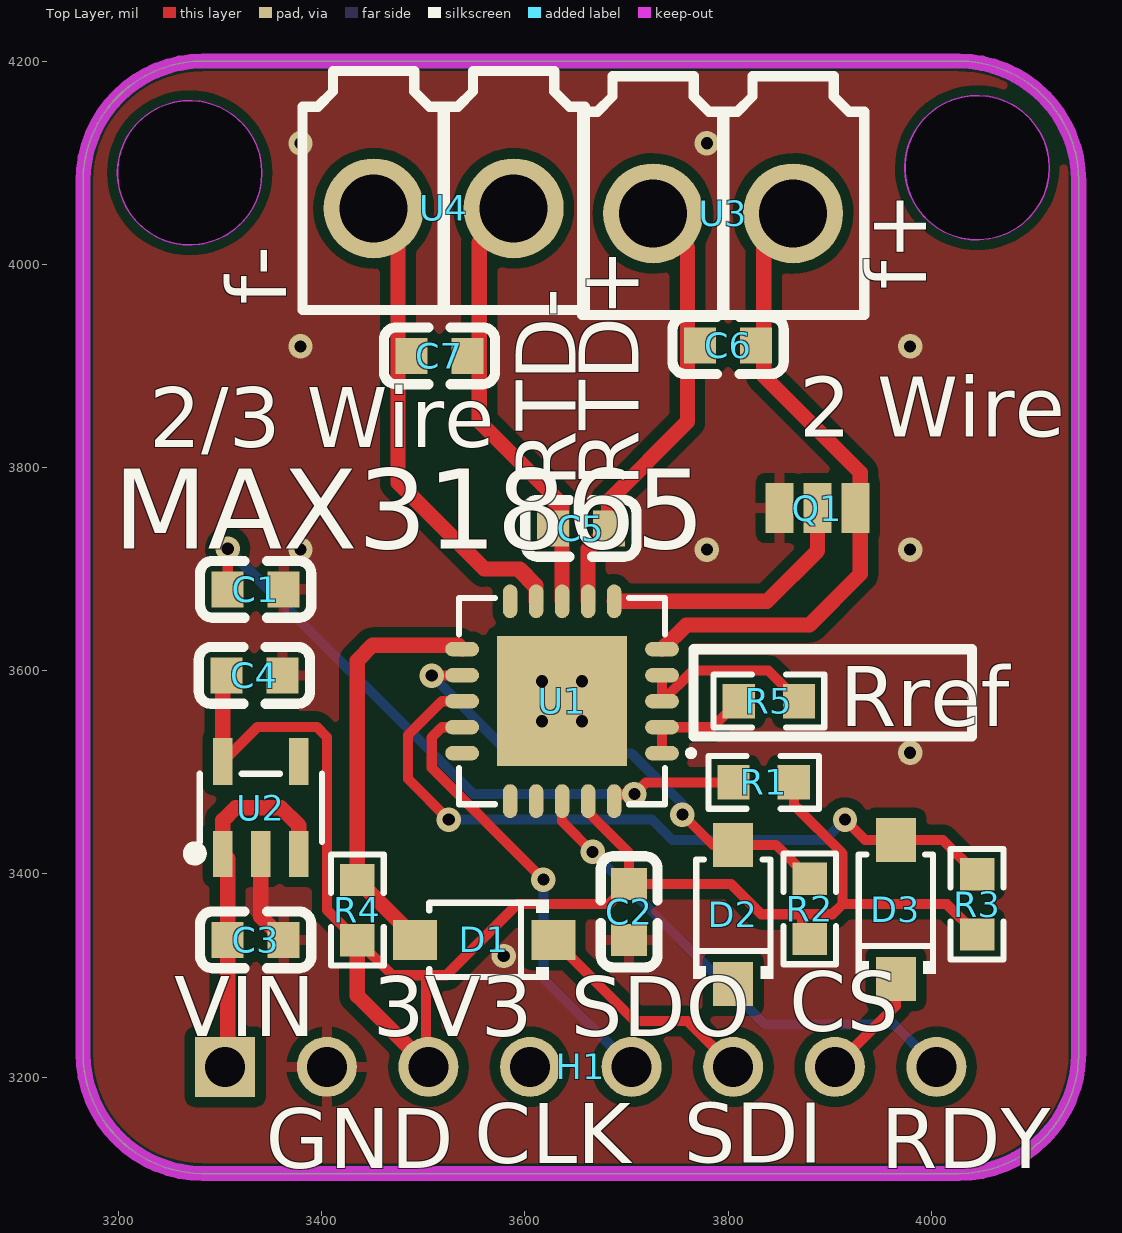
[diagram p0: Top Layer view]
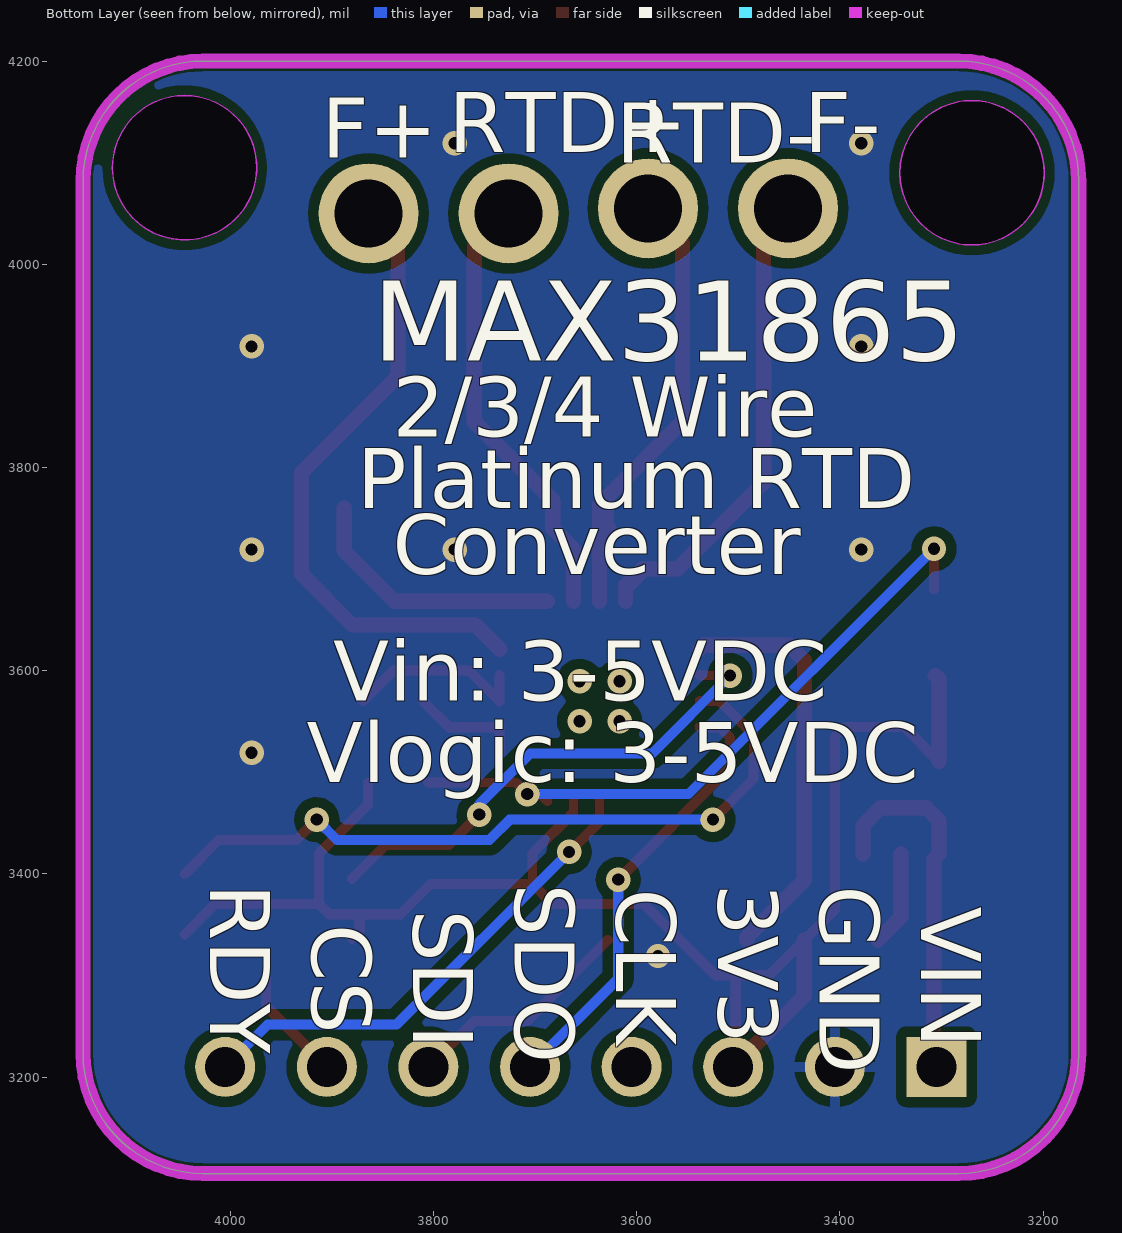
[diagram p1: Bottom Layer view, seen from below]
# Altium PCB MISC82906.pcbdoc
Units mil, origin at the board's own origin, x right, y up, seen from the top; angles counter-clockwise.
Board outline 980 x 1095 mil, 2 copper layers (Top Layer, Bottom Layer), stack 62.206 mil thick; 21 components, 20 nets, 71 pads, 21 vias.

## Layer stack, top to bottom
Top Solder Mask Layer: solder mask 0.394, Dk 3.3
Top Layer: signal copper 1.379
Dielectric1: surface 59.449, FR4, Dk 4.5
Bottom Layer: signal copper 1.378
Bottom Solder Mask Layer: solder mask 0.394, Dk 3.3

## Board outline
3283.11,4200 ccw(c3283.11,4081.89) 3165,4081.89 3165,3223.11 ccw(c3283.11,3223.11) 3283.11,3105 4026.89,3105 ccw(c4026.89,3223.11) 4145,3223.11 4145,4081.89 ccw(c4026.89,4081.89) 4026.89,4200
cut-out: 3341.06,4090 cw(c3270,4090) 3198.94,4090 cw(c3270,4090)
cut-out: 4116.06,4095 cw(c4045,4095) 3973.94,4095 cw(c4045,4095)

## Design rules (kind name [scope] priority, off if disabled: settings)
BoardOutlineClearance copperThickness2oz_1 [All] p2 off: genericclearance=7.99 ignorepadtopadclearanceinfootprint=FALSE except(0: Arc-SplitContinuation Track-SplitContinuation SMDPad-SplitContinuation THPad-SplitContinuation Via-SplitContinuation Fill-SplitContinuation Region-SplitContinuation Poly-SplitContinuation Text-SplitContinuation Hole-SplitContinuation; 5.98: Arc-CutoutEdge Track-CutoutEdge SMDPad-CutoutEdge THPad-CutoutEdge Via-CutoutEdge Text-CutoutEdge; 6.9: Hole-OutlineEdge Hole-CutoutEdge; 10: Poly-OutlineEdge Poly-CutoutEdge; 11.81: Arc-OutlineEdge Track-OutlineEdge SMDPad-OutlineEdge THPad-OutlineEdge Via-OutlineEdge Fill-OutlineEdge Region-OutlineEdge Text-OutlineEdge Fill-CutoutEdge Region-CutoutEdge)
BoardOutlineClearance Plane_innerPlane_1 [All] p4 off: genericclearance=4.02 ignorepadtopadclearanceinfootprint=FALSE except(0: Arc-SplitContinuation Track-SplitContinuation SMDPad-SplitContinuation THPad-SplitContinuation Via-SplitContinuation Fill-SplitContinuation Region-SplitContinuation Poly-SplitContinuation Text-SplitContinuation Hole-SplitContinuation; 5.98: Arc-CutoutEdge Track-CutoutEdge SMDPad-CutoutEdge THPad-CutoutEdge Via-CutoutEdge Text-CutoutEdge; 6.9: Hole-OutlineEdge Hole-CutoutEdge; 10: Poly-OutlineEdge Poly-CutoutEdge; 11.81: Arc-OutlineEdge Track-OutlineEdge SMDPad-OutlineEdge THPad-OutlineEdge Via-OutlineEdge Fill-OutlineEdge Region-OutlineEdge Text-OutlineEdge Fill-CutoutEdge Region-CutoutEdge)
BoardOutlineClearance Copper_copperRegion_1 [All] p6 off: genericclearance=4.02 ignorepadtopadclearanceinfootprint=FALSE except(0: Arc-SplitContinuation Track-SplitContinuation SMDPad-SplitContinuation THPad-SplitContinuation Via-SplitContinuation Fill-SplitContinuation Region-SplitContinuation Poly-SplitContinuation Text-SplitContinuation Hole-SplitContinuation; 5.98: Arc-CutoutEdge Track-CutoutEdge SMDPad-CutoutEdge THPad-CutoutEdge Via-CutoutEdge Text-CutoutEdge; 6.9: Hole-OutlineEdge Hole-CutoutEdge; 10: Poly-OutlineEdge Poly-CutoutEdge; 11.81: Arc-OutlineEdge Track-OutlineEdge SMDPad-OutlineEdge THPad-OutlineEdge Via-OutlineEdge Fill-OutlineEdge Region-OutlineEdge Text-OutlineEdge Fill-CutoutEdge Region-CutoutEdge)
BoardOutlineClearance copperThickness1oz_1 [All] p8: genericclearance=4.02 ignorepadtopadclearanceinfootprint=FALSE except(0: Arc-SplitContinuation Track-SplitContinuation SMDPad-SplitContinuation THPad-SplitContinuation Via-SplitContinuation Fill-SplitContinuation Region-SplitContinuation Poly-SplitContinuation Text-SplitContinuation Hole-SplitContinuation; 5.98: Arc-CutoutEdge Track-CutoutEdge SMDPad-CutoutEdge THPad-CutoutEdge Via-CutoutEdge Text-CutoutEdge; 6.9: Hole-OutlineEdge Hole-CutoutEdge; 10: Poly-OutlineEdge Poly-CutoutEdge; 11.81: Arc-OutlineEdge Track-OutlineEdge SMDPad-OutlineEdge THPad-OutlineEdge Via-OutlineEdge Fill-OutlineEdge Region-OutlineEdge Text-OutlineEdge Fill-CutoutEdge Region-CutoutEdge)
Clearance copperThickness2oz [All] p1 off: gap=7.99 ignorepadtopadclearanceinfootprint=FALSE except(5.98: SMDPad-Track SMDPad-SMDPad THPad-Track SMDPad-THPad THPad-THPad Track-Via SMDPad-Via THPad-Via Via-Via Fill-SMDPad Region-SMDPad Fill-THPad Region-THPad Fill-Via Region-Via Fill-Fill Fill-Region Region-Region Arc-Track Arc-SMDPad Arc-THPad Arc-Via Fill-Arc Region-Arc Arc-Arc Text-Track SMDPad-Text Text-THPad Text-Via Fill-Text Region-Text Arc-Text Text-Text; 6.9: Hole-Track Hole-SMDPad Hole-THPad Hole-Via Fill-Hole Region-Hole Hole-Arc Hole-Text; 10: Poly-Track Poly-SMDPad Poly-THPad Poly-Via Poly-Fill Poly-Region Poly-Poly Poly-Arc Poly-Text Poly-Hole; 11.81: Fill-Track Region-Track)
Clearance Plane_innerPlane [All] p3 off: gap=4.02 ignorepadtopadclearanceinfootprint=FALSE except(5.98: SMDPad-Track SMDPad-SMDPad THPad-Track SMDPad-THPad THPad-THPad Track-Via SMDPad-Via THPad-Via Via-Via Fill-SMDPad Region-SMDPad Fill-THPad Region-THPad Fill-Via Region-Via Fill-Fill Fill-Region Region-Region Arc-Track Arc-SMDPad Arc-THPad Arc-Via Fill-Arc Region-Arc Arc-Arc Text-Track SMDPad-Text Text-THPad Text-Via Fill-Text Region-Text Arc-Text Text-Text; 6.9: Hole-Track Hole-SMDPad Hole-THPad Hole-Via Fill-Hole Region-Hole Hole-Arc Hole-Text; 10: Poly-Track Poly-SMDPad Poly-THPad Poly-Via Poly-Fill Poly-Region Poly-Poly Poly-Arc Poly-Text Poly-Hole; 11.81: Fill-Track Region-Track)
Clearance Copper_copperRegion [All] p5 off: gap=4.02 ignorepadtopadclearanceinfootprint=FALSE except(5.98: SMDPad-Track SMDPad-SMDPad THPad-Track SMDPad-THPad THPad-THPad Track-Via SMDPad-Via THPad-Via Via-Via Fill-SMDPad Region-SMDPad Fill-THPad Region-THPad Fill-Via Region-Via Fill-Fill Fill-Region Region-Region Arc-Track Arc-SMDPad Arc-THPad Arc-Via Fill-Arc Region-Arc Arc-Arc Text-Track SMDPad-Text Text-THPad Text-Via Fill-Text Region-Text Arc-Text Text-Text; 6.9: Hole-Track Hole-SMDPad Hole-THPad Hole-Via Fill-Hole Region-Hole Hole-Arc Hole-Text; 10: Poly-Track Poly-SMDPad Poly-THPad Poly-Via Poly-Fill Poly-Region Poly-Poly Poly-Arc Poly-Text Poly-Hole; 11.81: Fill-Track Region-Track)
Clearance copperThickness1oz [All] p7: gap=4.02 ignorepadtopadclearanceinfootprint=FALSE except(5.98: SMDPad-Track SMDPad-SMDPad THPad-Track SMDPad-THPad THPad-THPad Track-Via SMDPad-Via THPad-Via Via-Via Fill-SMDPad Region-SMDPad Fill-THPad Region-THPad Fill-Via Region-Via Fill-Fill Fill-Region Region-Region Arc-Track Arc-SMDPad Arc-THPad Arc-Via Fill-Arc Region-Arc Arc-Arc Text-Track SMDPad-Text Text-THPad Text-Via Fill-Text Region-Text Arc-Text Text-Text; 6.9: Hole-Track Hole-SMDPad Hole-THPad Hole-Via Fill-Hole Region-Hole Hole-Arc Hole-Text; 10: Poly-Track Poly-SMDPad Poly-THPad Poly-Via Poly-Fill Poly-Region Poly-Poly Poly-Arc Poly-Text Poly-Hole; 11.81: Fill-Track Region-Track)
DiffPairsRouting differentialPair [All] p1: maxlimit=6 minlimit=6 mostfreqgap=6 toplayer_minwidth=5 toplayer_prefwidth=10 toplayer_maxwidth=100 toplayer_mingap=6 toplayer_prefgap=6 toplayer_maxgap=6 bottomlayer_minwidth=5 bottomlayer_prefwidth=10 bottomlayer_maxwidth=100 bottomlayer_mingap=6 bottomlayer_prefgap=6 bottomlayer_maxgap=6 maxuncoupledlength=10
HoleToHoleClearance otherClearance [All] p1: gap=11.81 allowstackedmicrovias=TRUE
Length netLength [All] p1: minlimit=0 maxlimit=0
PasteMaskExpansion pasteMaskExpansion [All] p1: expansion=0
PlaneConnect innerPlane [All] p1: planeconnectstyle=Relief reliefexpansion=20 reliefentries=4 reliefconductorwidth=10 reliefairgap=10
PolygonConnect copperRegion [All] p1: connectstyle=Relief reliefconductorwidth=10 reliefentries=4 polygonreliefangle="90 Angle" airgapwidth=10 via.connectstyle=Relief via.reliefconductorwidth=10 via.reliefentries=4 via.polygonreliefangle="90 Angle" via.airgapwidth=10
RoutingVias viaSize [All] p1: holewidth=12.01 width=24.02 viastyle="Through Hole" minholewidth=11.81 minwidth=19.68 maxholewidth=248.03 maxwidth=393.7
SolderMaskExpansion solderMaskExpansion [IsVia] p1: expansion=-1000 istentingtop=TRUE
SolderMaskExpansion solderMaskExpansion [All] p2: expansion=2 istentingtop=FALSE
Width copperThickness2oz_2 [All] p1 off: maxlimit=100 minlimit=8 preferedwidth=10
Width copperThickness1oz_2 [All] p2: maxlimit=100 minlimit=5 preferedwidth=10

## Components (designator, comment, footprint, x,y, rotation, side; value= is the part's Value field where it differs from the comment)
C1 "100nF" C0603 3335,3680 r180 top
C2 "100nF" C0603 3702.56,3362.56 r90 top
C3 "10uF" C0603 3335,3335 r180 top
C4 "10uF" C0603 3333.72,3595.27 r180 top
C5 "100nF" C0603 3655,3740 r0 top
C6 "100nF" C0603 3800,3920 r0 top
C7 "100nF" C0603 3515.86,3909.81 r0 top
D1 "1N4148W" SOD-123F_L2.7-W1.6-LS3.8-RD 3560,3335 r180 top
D2 "1N4148W" SOD-123F_L2.7-W1.6-LS3.8-RD 3805,3360 r90 top
D3 "1N4148W" SOD-123F_L2.7-W1.6-LS3.8-RD 3965,3365 r90 top
H1 "" HDR-TH_8P-P2.54-V-M 3655,3210 r0 top
Q1 "" S8550P_SOT 3887.9,3759.12 r90 top
R1 "10K" R0603 3835,3490 r0 top
R2 "10K" R0603 3880.32,3365.51 r270 top
R3 "10K" R0603 4045,3370 r270 top
R4 "10K" R0603 3435,3364.32 r270 top
R5 "10K" R0603 3840,3570 r180 top
U1 "MAX3186" QFN-20_L5.0-W5.0-P0.65-BL-EP 3636.54,3569.89 r90 top
U2 "MIC5225-3.3" SOT-23-5_L3.0-W1.7-P0.95-LS2.8-BL 3340,3465 r0 top
U3 "KF2EDGJVC-3.5-2P" CONN-TH_2P-P3.50_KEFA_KF2EDGJVC-3.5-2P 3795,4050 r0 top
U4 "KF2EDGJVC-3.5-2P" CONN-TH_2P-P3.50_KEFA_KF2EDGJVC-3.5-2P 3520,4055 r0 top

## Footprints (in the part's own frame and the unit in brackets; to place one, negate y for a bottom-side part, rotate by r counter-clockwise, add the part's x,y. Pads: shape width x height; smd on the part's side, far side on the other; paste and mask are expansions set on the pad)
C0603 [mm]
  rect 0.8x0.9 smd: 1(-0.7,0) 2(0.7,0)
  silkscreen extent -1.39,-0.71 1.39,0.71
CONN-TH_2P-P3.50_KEFA_KF2EDGJVC-3.5-2P [mm]
  round 2.5 hole 1.7 paste+0 mask+0.05: 1(-1.75,0) 2(1.75,0)
  silkscreen extent -3.53,-2.54 3.53,3.43
HDR-TH_8P-P2.54-V-M [mm]
  rect 1.5x1.5 hole 1: 1(-8.89,0)
  round 1.5 hole 1: 2(-6.35,0) 3(-3.81,0) 4(-1.27,0) 5(1.27,0) 6(3.81,0) 7(6.35,0) 8(8.89,0)
QFN-20_L5.0-W5.0-P0.65-BL-EP [mm]
  oval 0.364x0.847 smd: 1(-1.3,-2.499) 2(-0.65,-2.499) 3(0,-2.499) 4(0.65,-2.499) 5(1.3,-2.499) 11(1.3,2.499) 12(0.65,2.499) 13(0,2.499) 14(-0.65,2.499) 15(-1.3,2.499)
  oval 0.847x0.364 smd: 6(2.499,-1.3) 7(2.499,-0.65) 8(2.499,0) 9(2.499,0.65) 10(2.499,1.3) 16(-2.499,1.3) 17(-2.499,0.65) 18(-2.499,0) 19(-2.499,-0.65) 20(-2.499,-1.3)
  rect 3.25x3.25 smd: 21(0,0)
  silkscreen extent -2.58,-3.3 2.58,2.58
R0603 [mil]
  rect 31.75x34.02 smd paste-3937.01 mask+2: 1(-29.66,0) 2(29.66,0)
  silkscreen extent -55,-26 55,26
S8550P_SOT [mil]
  rect 49.2x27.6 smd paste+0 mask+2: 1(0.84,0) 2(0.84,37.4) 3(0.84,-37.4)
SOD-123F_L2.7-W1.6-LS3.8-RD [mm]
  rect 1.1x1 smd: 1(-1.735,0) 2(1.735,0)
  silkscreen extent -1.6,-1 1.38,1
SOT-23-5_L3.0-W1.7-P0.95-LS2.8-BL [mm]
  rect 0.49x1.157 smd: 1(-0.95,-1.154) 2(0,-1.154) 3(0.95,-1.154)
  rect 0.49x1.175 smd: 4(0.95,1.154) 5(-0.95,1.154)
  silkscreen extent -1.8,-1.29 1.53,0.85

## Via types
v1: diameter 24.02, hole 12, Top Layer to Bottom Layer, 17 vias
v2: diameter 24, hole 12, Top Layer to Bottom Layer, 4 vias

## Nets (pads, with @x,y where several pads share a name; then routed paths per layer and width w, separated by ;. In a path a pad name is that pad's centre, name@x,y a point inside that pad or via, vN(x,y) a via of type N, cw(c..) or ccw(c..) an arc to the next point about the centre after c; other vN are vias at no path point)
$1N345: C1.2 R1.1 U1.20 | length 665.6
  Top Layer w10: C1.2 v1(3307.44,3720) ; U1.20 3694.68,3478.48 v1(3707.72,3478.48) 3719.24,3490 R1.1
  Bottom Layer w10: v1(3307.44,3720) 3548.96,3478.48 v1(3707.72,3478.48)
$1N719: D1.2 R4.1 U1.11 | length 409.5
  Top Layer w15: D1.2 3491.7,3337.28 R4.1 3435,3610 3450,3625 3534.24,3625 U1.11
$1N723: D2.2 R2.1 U1.12 | length 491
  Top Layer w10: v1(3508.17,3595.13) 3537.82,3595.13 U1.12 ; v1(3755,3458.3) 3785,3428.3 D2.2 3847.18,3428.3 R2.1
  Bottom Layer w10: v1(3508.17,3595.13) 3585,3518.3 3705,3518.3 3755,3468.3 v1(3755,3458.3)
$1N730: D3.2 R3.1 U1.13 | length 725.7
  Top Layer w10: v1(3525,3453.3) 3485,3493.3 3485,3536.72 3518.17,3569.89 U1.13 ; v1(3915,3453.3) 3935,3433.3 D3.2 4011.36,3433.3 R3.1
  Bottom Layer w10: v1(3525,3453.3) 3725,3453.3 3745,3433.3 3895,3433.3 v1(3915,3453.3)
$1N1605: R5.2 U1.1 U1.2 | length 111.7
  Top Layer w10: U1.1 U1.2 3784.64,3544.3 R5.2
$1N1645: R5.1 U1.3 U1.4 | length 185.2
  Top Layer w10: U1.4 U1.3 3765.02,3600 3839.66,3600 R5.1
$1N1753: C6.2 Q1.3 U1.5 U3.2 | length 632
  Top Layer w15: U1.5 3758.84,3645 3880,3645 3930,3695 3930,3795 3835,3890 3835,4021.1 U3.2
$1N1757: C5.1 C7.2 U1.8 U4.2 | length 480
  Top Layer w10: C5.1 3627.44,3772.56
  Top Layer w15: U4.2 3555,4021.1 3555,3845 3627.44,3772.56 3636.54,3763.46 C5.1@3636.54,3730.9 ; C5.1 C5.1@3636.54,3730.9 ; U1.8 C5.1@3636.54,3730.9
$1N1762: C5.2 C6.1 U1.7 U3.1 | length 436.3
  Top Layer w15: U1.7 3662.13,3719.57 C5.2 3682.56,3767.56 3760,3845 3760,4016.1 U3.1
$1N1808: C7.1 U1.9 U4.1 | length 504.2
  Top Layer w10: 3589.21,3700 U1.9@3610.95,3678.26
  Top Layer w15: U4.1 3475,4031.1 3475,3785 3560,3700 3589.21,3700 3595,3700 3610.95,3684.05 3610.95,3678.26 U1.9
$1N2395: Q1.1 U1.6 | length 262.8
  Top Layer w15: U1.6 3838.26,3668.26 3887.9,3717.9 Q1.1
CS_5V: D3.1 H1.7 | length 111.5
  Top Layer w10: H1.7 3965,3270 D3.1
DRDY: H1.8 U1.18 | length 488.5
  Top Layer w10: U1.18 3636.54,3451.52 v1(3666.54,3421.52)
  Bottom Layer w10: v1(3666.54,3421.52) 3836.54,3251.52 3963.48,3251.52 H1.8
GND: C1.1 C2.1 C3.1 C4.1 H1.2 Q1.2 U2.2 | length 93.9
  Top Layer w15: U2.2 3340,3357.56 C3.1
  other v1: 3579.1,3319.1 3979.1,3519.1 3379.1,3719.1 3779.1,3719.1 3979.1,3719.1 3379.1,3919.1 3979.1,3919.1 3379.1,4119.1 3779.1,4119.1
SCI_K_5V: D2.1
SCL_K_5V: H1.4
SD0: H1.5 U1.14 | length 440
  Top Layer w10: U1.14 3518.17,3544.3 3508.17,3534.3 3508.17,3504.3 v1(3618.17,3394.3)
  Bottom Layer w10: v1(3618.17,3394.3) 3618.17,3296.83 H1.5
SDI_5V: D1.1 H1.6 | length 228.5
  Top Layer w10: D1.1 3708.3,3255 3760,3255 H1.6
VDD: C2.2 C4.2 H1.3 R1.2 R2.2 R3.2 R4.2 U1.19 U2.5 | length 1616.7
  Top Layer w10: U2.5 3336.84,3544.66 3395,3544.66 3405,3534.66 3405,3364.66 R4.2 3469.54,3300.12 3502.56,3300.12 ; H1.3@3502.56,3212.44 3502.56,3300.12 ; U1.19 3662.13,3460.55 3702.56,3420.12 C2.2 ; R1.2 3864.66,3468.02 3912.56,3420.12 3912.56,3370.12 ; R2.2 3872.56,3343.6 3872.56,3360.12 ; R3.2 4015.22,3370.12 3912.56,3370.12 ; 3502.56,3300.12 3522.56,3300.12 3592.56,3370.12 3682.56,3370.12 C2.2 ; C2.2 3802.56,3390.12 3832.56,3360.12 3872.56,3360.12 ; 3872.56,3360.12 3902.56,3360.12 3912.56,3370.12
  Top Layer w15: U2.5 3302.6,3591.72 C4.2 ; R4.2 3435,3280 3502.56,3212.44 H1.3
VIN: C3.2 H1.1 U2.1 U2.3 | length 376.2
  Top Layer w10: U2.3 U2.3@3377.44,3435
  Top Layer w15: H1.1 3307.44,3212.44 C3.2 3307.44,3414.74 U2.1 3302.6,3452.6 3315,3465 3360,3465 3377.4,3447.6 3377.4,3435.04 U2.3
pads on no net: U1.10 U1.15 U1.16 U1.17 U1.21 U2.4
copper on no net:
  other v2: 3616.86,3550.2 3656.23,3550.2 3616.86,3589.58 3656.23,3589.58

## Polygon pours and split planes (outlines as drawn)
GND on Top Layer (solid, remove dead copper, pour order 0): 3005,4350 3005,3035 4270,3035 4270,4350
GND on Bottom Layer (solid, remove dead copper, pour order 2): 3000,4365 3000,3000 4240,3000 4240,4365

## Keep-outs
Board Outline Layer:
  region: 3341.06,4090 cw(c3270,4090) 3198.94,4090 cw(c3270,4090)
  circle w0.1: c3270,4090 r71.06
  region: 3341.06,4090 3340.67,4082.57 3339.51,4075.23 3337.59,4068.04 3334.92,4061.1 3331.54,4054.47 3327.49,4048.23 3322.81,4042.45 3317.55,4037.19 3311.77,4032.51 3305.53,4028.46 3298.9,4025.08 3291.96,4022.41 3284.77,4020.49 3277.43,4019.33 3270,4018.94 3262.57,4019.33 3255.23,4020.49 3248.04,4022.41 3241.1,4025.08 3234.47,4028.46 3228.23,4032.51 3222.45,4037.19 3217.19,4042.45 3212.51,4048.23 3208.46,4054.47 3205.08,4061.1 3202.41,4068.04 3200.49,4075.23 3199.33,4082.57 3198.94,4090 3199.33,4097.43 3200.49,4104.77 3202.41,4111.96 3205.08,4118.9 3208.46,4125.53 3212.51,4131.77 3217.19,4137.55 3222.45,4142.81 3228.23,4147.49 3234.47,4151.54 3241.1,4154.92 3248.04,4157.59 3255.23,4159.51 3262.57,4160.67 3270,4161.06 3277.43,4160.67 3284.77,4159.51 3291.96,4157.59 3298.9,4154.92 3305.53,4151.54 3311.77,4147.49 3317.55,4142.81 3322.81,4137.55 3327.49,4131.77 3331.54,4125.53 3334.92,4118.9 3337.59,4111.96 3339.51,4104.77 3340.67,4097.43
  region: 4116.06,4095 cw(c4045,4095) 3973.94,4095 cw(c4045,4095)
  circle w0.1: c4045,4095 r71.06
  region: 4116.06,4095 4115.67,4087.57 4114.51,4080.23 4112.59,4073.04 4109.92,4066.1 4106.54,4059.47 4102.49,4053.23 4097.81,4047.45 4092.55,4042.19 4086.77,4037.51 4080.53,4033.46 4073.9,4030.08 4066.96,4027.41 4059.77,4025.49 4052.43,4024.33 4045,4023.94 4037.57,4024.33 4030.23,4025.49 4023.04,4027.41 4016.1,4030.08 4009.47,4033.46 4003.23,4037.51 3997.45,4042.19 3992.19,4047.45 3987.51,4053.23 3983.46,4059.47 3980.08,4066.1 3977.41,4073.04 3975.49,4080.23 3974.33,4087.57 3973.94,4095 3974.33,4102.43 3975.49,4109.77 3977.41,4116.96 3980.08,4123.9 3983.46,4130.53 3987.51,4136.77 3992.19,4142.55 3997.45,4147.81 4003.23,4152.49 4009.47,4156.54 4016.1,4159.92 4023.04,4162.59 4030.23,4164.51 4037.57,4165.67 4045,4166.06 4052.43,4165.67 4059.77,4164.51 4066.96,4162.59 4073.9,4159.92 4080.53,4156.54 4086.77,4152.49 4092.55,4147.81 4097.81,4142.55 4102.49,4136.77 4106.54,4130.53 4109.92,4123.9 4112.59,4116.96 4114.51,4109.77 4115.67,4102.43
  lines w15: 3165,3223.11 3165,4081.89 cw(c3283.11,4081.89) 3283.11,4200 4026.89,4200 cw(c4026.89,4081.89) 4145,4081.89 4145,3223.11 cw(c4026.89,3223.11) 4026.89,3105 3283.11,3105 cw(c3283.11,3223.11) 3165,3223.11

## Silkscreen, mask and mechanical layers (free items; w line width, h text height)
Top Silkscreen Layer:
  lines w10: 3765.94,3535 3765.94,3621.07 4040,3621.07 4040,3535 3765.94,3535
  text "f+" at 3995,3975 h59.06 r90
  text "f-" at 3365,3960 h59.06 r90
  text "2 Wire" at 3870,3830 h59.06
  text "2/3 Wire" at 3230,3820 h59.06
  text "RTD+" at 3712.09,3780.53 h59.06 r90
  text "RTD-" at 3650,3780 h59.06 r90
  text "MAX31865" at 3195,3720 h78.74
  text "Rref" at 3910,3545 h59.06
  text "CS" at 3860,3245 h59.06
  text "VIN" at 3255,3240 h59.06
  text "3V3" at 3450,3240 h59.06
  text "SDO" at 3645,3240 h59.06
  text "CLK" at 3550,3115 h59.06
  text "SDI" at 3756.4,3115.47 h59.06
  text "GND" at 3345,3110 h59.06
  text "RDY" at 3950,3110 h59.06
Bottom Silkscreen Layer:
  text "F-" at 3435,4110 h59.06
  text "RTD+" at 3785,4110 h59.06
  text "F+" at 3910,4105 h59.06
  text "RTD-" at 3620,4100 h59.06
  text "MAX31865" at 3860,3905 h78.74
  text "2/3/4 Wire" at 3840,3830 h59.06
  text "Platinum RTD" at 3875,3760 h59.06
  text "Converter" at 3840,3695 h59.06
  text "Vin: 3-5VDC" at 3898.85,3570.47 h59.06
  text "Vlogic: 3-5VDC" at 3925,3490 h59.06
  text "3V3" at 3520,3390 h59.06 r90
  text "SDO" at 3720,3390 h59.06 r90
  text "RDY" at 4020,3390 h59.06 r90
  text "GND" at 3420,3388.4 h59.06 r90
  text "CLK" at 3620,3385.2 h59.06 r90
  text "VIN" at 3320,3367.7 h59.06 r90
  text "SDI" at 3820,3364.5 h59.06 r90
  text "CS" at 3920,3350.4 h59.06 r90
Mechanical Layer:
  circle w0.1: c3270,4090 r71.06
  circle w0.1: c4045,4095 r71.06